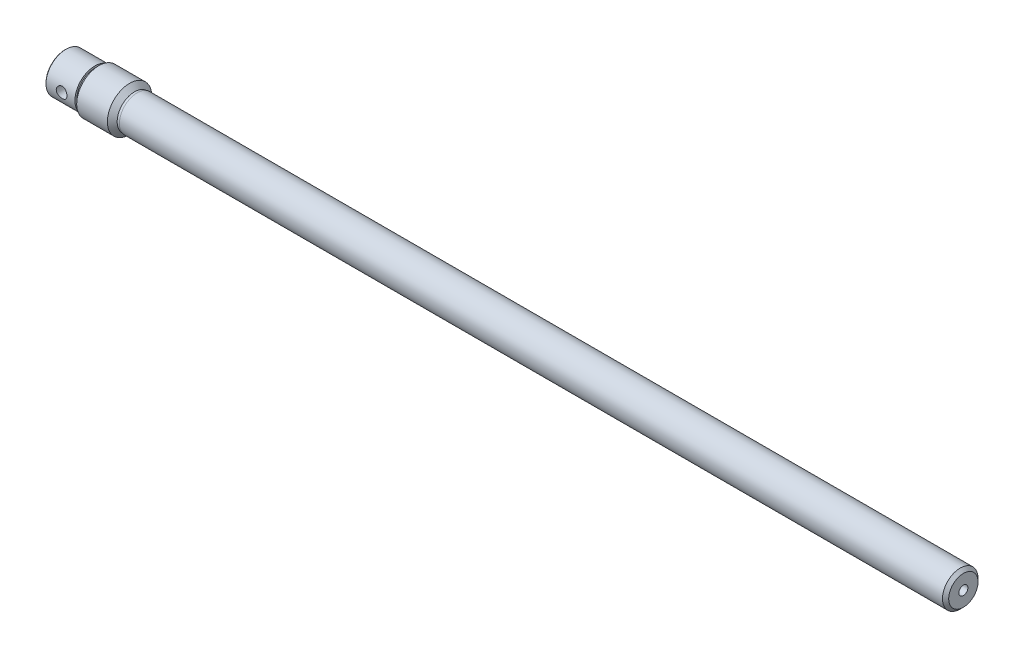
SolidWorks part; units mm, degrees
ref_plane "Front Plane" through (0, 0, 0) normal (0, 0, 1) x (1, 0, 0)
ref_plane "Top Plane" through (0, 0, 0) normal (0, 1, 0) x (1, 0, 0)
ref_plane "Right Plane" through (0, 0, 0) normal (1, 0, 0) x (0, 0, -1)
sketch "Sketch1" plane through (0, 0, 0) normal (0, 0, 1) x (1, 0, 0)
  line L0 (78, 19.5) -> (72.5, 25)
  line L5 (0, 0) -> (38, 0)
  line L6 (0, 0) -> (0, 22.5)
  line L7 (0, 22.5) -> (38, 22.5)
  line L8 (38, 20.3) -> (38, 22.5)
  line L9 (38, 0) -> (78, 0)
  line L10 (38, 20.3) -> (38, 25)
  line L11 (38, 25) -> (72.5, 25)
  line L12 (78, 0) -> (78, 19.5) construction
  line L13 (78, 0) -> (81, 0)
  line L14 (78, 0) -> (78, 19.5) construction
  line L15 (78, 19.5) -> (81, 19.5)
  line L16 (81, 0) -> (81, 19.5) construction
  line L17 (81, 0) -> (1010, 0)
  line L18 (81, 19.5) -> (81, 20)
  line L19 (81, 20) -> (1010, 20)
  line L20 (1010, 0) -> (1010, 20)
  line L21 (38, 22.5) -> (33.5, 22.5)
  line L22 (38, 22.5) -> (38, 20.3)
  line L23 (38, 20.3) -> (33.5, 20.3)
  line L24 (33.5, 22.5) -> (33.5, 20.3)
  line L25 (78, 19.5) -> (78, 25) construction
  line L26 (72.5, 25) -> (78, 25) construction
  line L27 (81, 0) -> (81, 19.5) construction
  line L28 (38, 0) -> (38, 20.3) construction
  line L29 (38, 0) -> (38, 20.3) construction
  dimension "D1" = 22.5
  dimension "D2" = 38
  dimension "D3" = 25
  dimension "D4" = 78
  dimension "D5" = 19.5
  dimension "D6" = 3
  dimension "D7" = 20
  dimension "D8" = 1010
  dimension "D9" = 20.3
  dimension "D10" = 4.5
  dimension "D11" = 45
revolve "Revolve1" add sketch "Sketch1" angle 360 about L9
cosmetic thread "Cosmetic Thread1" parameters "D2"=40.129
chamfer "Chamfer1" distance 3.5 angle 45 1 edges at (1010, 0, 20)
chamfer "Chamfer2" distance 1 angle 45 1 edges at (0, 0, 22.5)
sketch "Sketch2" plane through (0, 0, 0) normal (0, 0, 1) x (1, 0, 0)
  line L0 (0, 0) -> (18.5, 0) construction
  circle A0 centre (18.5, 0) radius 6
  dimension "D2" = 12
  dimension "D1" = 18.5
extrude "Cut-Extrude1" cut sketch "Sketch2" against normal mid plane 100
hole_wizard "M12 Tapped Hole1" positions "Sketch3" profile "Sketch5" tap size "M12" standard "GB"
sketch "Sketch3" plane through (1010, 0, 0) normal (1, 0, 0) x (0, 0, -1)
  point P0 (0, 0)
sketch "Sketch5" plane through (1010, 0, 0) normal (0, 1, 0) x (0, 0, -1)
  line L0 (0, 0) -> (0, 26.3144)
  line L1 (0, 26.3144) -> (5.1, 23.25)
  line L2 (5.1, 23.25) -> (5.1, 0)
  line L5 (5.1, 0) -> (0, 0)
  line L10 (0, 26.3144) -> (-5.1, 23.25) construction
  line L11 (0, -6.35) -> (0, 107.95) construction
  dimension "螺纹孔钻头直径" = 10.2
  dimension "螺纹孔钻头深度" = 23.25
  dimension "导头角度" = 118
cosmetic thread "孔螺纹线1" parameters "D1"=18, "D2"=12
